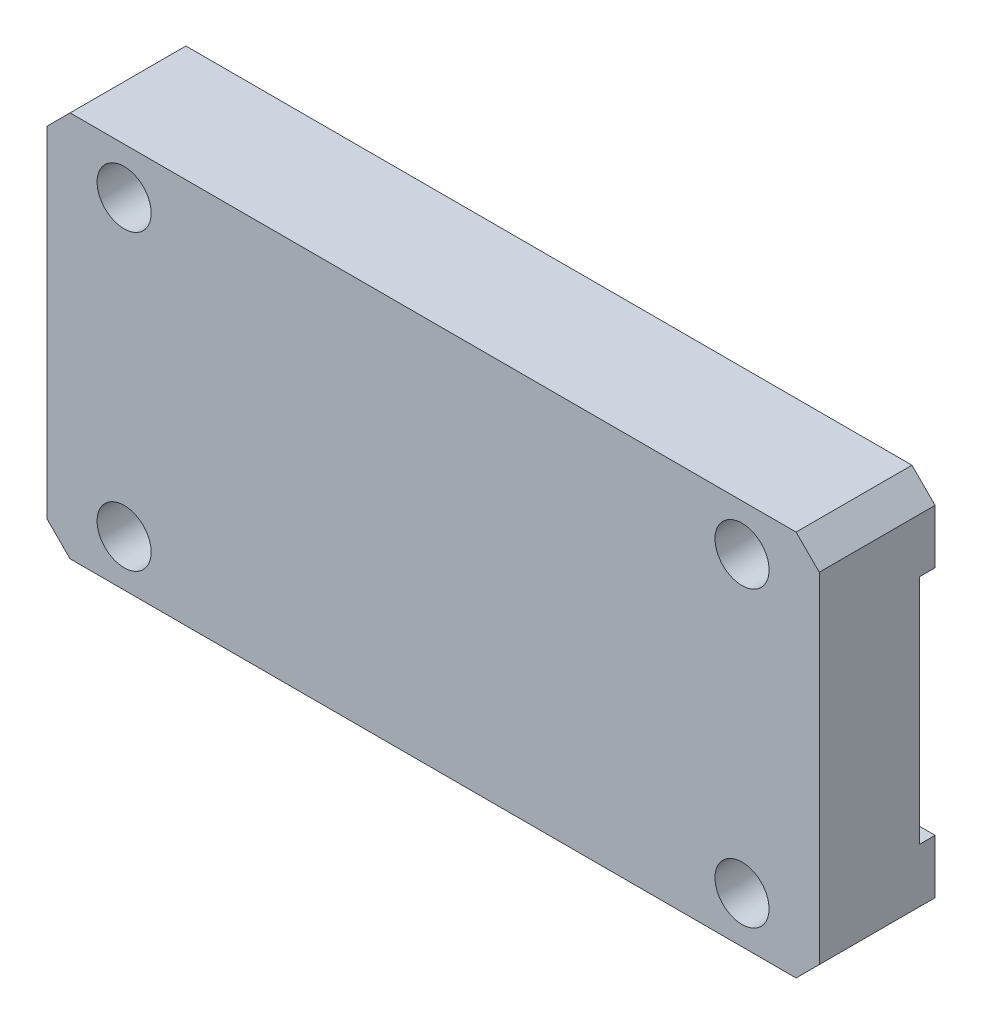
SolidWorks part; units mm, degrees
ref_plane "前视基准面" through (0, 0, 0) normal (0, 0, 1) x (1, 0, 0)
ref_plane "上视基准面" through (0, 0, 0) normal (0, 1, 0) x (1, 0, 0)
ref_plane "右视基准面" through (0, 0, 0) normal (1, 0, 0) x (0, 0, -1)
sketch "草图1" plane through (0, 0, 0) normal (0, 0, 1) x (1, 0, 0)
  line L1 (0, 0) -> (100, 0)
  line L2 (0, 0) -> (0, 50)
  line L3 (0, 50) -> (100, 50)
  line L4 (100, 0) -> (100, 50)
  dimension "D1" = 100
  dimension "D2" = 50
extrude "凸台-拉伸1" add sketch "草图1" along normal blind 15
hole_wizard "Ø7.0 (7) 直径孔1" positions "草图3" profile "草图2" hole size "Ø7.0" standard "GB" end condition through all
sketch "草图3" plane through (0, 0, 0) normal (0, 0, -1) x (-1, 0, 0)
  line L0 (-50, 50) -> (-50, -13.8627) construction
  line L1 (-100, 50) -> (0, 50) construction
  line L3 (0, 25) -> (-128.1116, 25) construction
  line L4 (0, 50) -> (0, 0) construction
  point P0 (-10, 44)
  point P3 (-10, 6)
  point P6 (-90, 44)
  point P9 (-90, 6)
  dimension "D1" = 80
  dimension "D2" = 38
sketch "草图2" plane through (10, 44, 0) normal (1, 0, 0) x (0, 1, 0)
  line L0 (0, 0) -> (0, 15)
  line L1 (0, 15) -> (3.5, 15)
  line L2 (3.5, 15) -> (3.5, 0)
  line L5 (3.5, 0) -> (0, 0)
  line L11 (0, -6.35) -> (0, 107.95) construction
  dimension "通孔孔直径" = 7
  dimension "通孔孔深度" = 15
chamfer "倒角1" distance 3 angle 45 4 edges at (0, 0, 7.5) (0, 50, 7.5) (100, 0, 7.5) (100, 50, 7.5)
sketch "草图6" plane through (0, 0, 0) normal (-1, 0, 0) x (0, 0, 1)
  line L0 (0, 47) -> (0, 3) construction
  line L1 (0, 40) -> (2, 40)
  line L2 (0, 40) -> (0, 10)
  line L3 (0, 10) -> (2, 10)
  line L4 (2, 40) -> (2, 10)
  line L5 (15, 25) -> (-4.0845, 25) construction
  line L6 (15, 47) -> (15, 3) construction
  dimension "D1" = 2
  dimension "D2" = 30
extrude "切除-拉伸1" cut sketch "草图6" against normal blind 113
